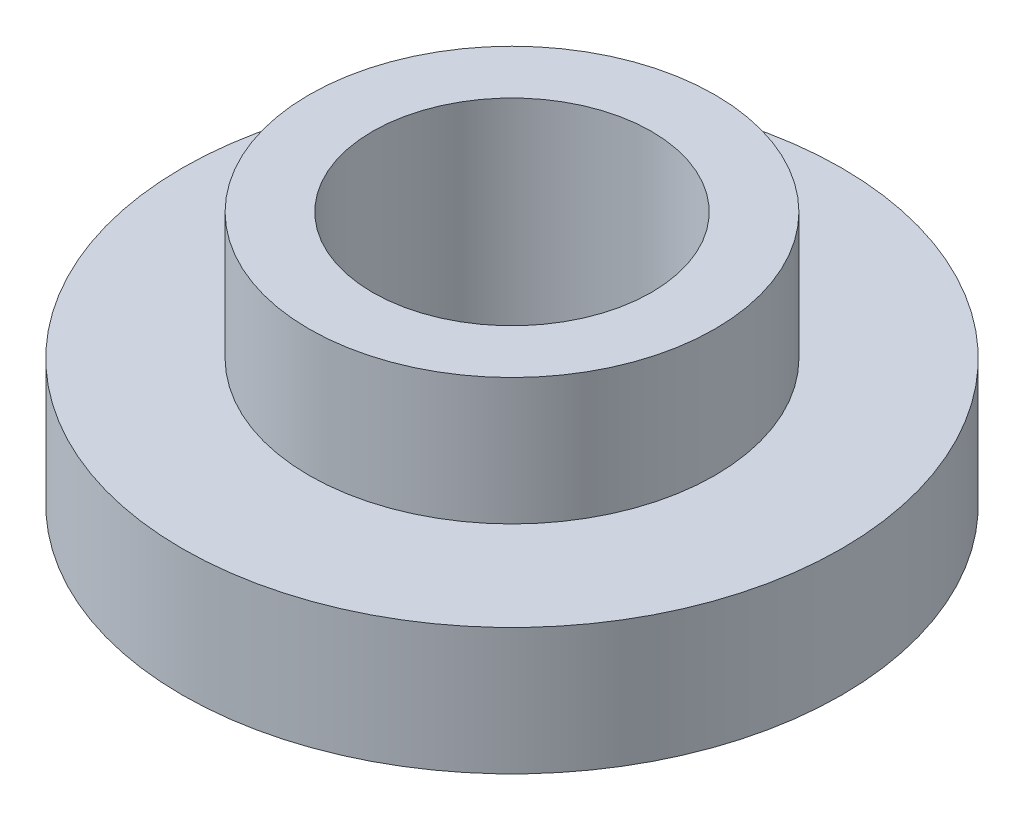
SolidWorks part; units mm, degrees
ref_plane "Front Plane" through (0, 0, 0) normal (0, 0, 1) x (1, 0, 0)
ref_plane "Top Plane" through (0, 0, 0) normal (0, 1, 0) x (1, 0, 0)
ref_plane "Right Plane" through (0, 0, 0) normal (1, 0, 0) x (0, 0, -1)
sketch "Sketch1" plane through (0, 0, 0) normal (0, 0, 1) x (1, 0, 0)
  line L0 (-29.5, 0) -> (-65, 0)
  line L1 (-65, 0) -> (-65, 25)
  line L2 (-65, 25) -> (-40, 25)
  line L3 (-40, 25) -> (-40, 50)
  line L4 (-40, 50) -> (-27.5, 50)
  line L5 (-27.5, 50) -> (-27.5, 2)
  line L6 (0, 0) -> (0, 42.4846) construction
  line L7 (0, 0) -> (-27.5, 0) construction
  line L8 (-27.5, 2) -> (-29.5, 0)
  dimension "D1" = 130
  dimension "D2" = 80
  dimension "D3" = 55
  dimension "D4" = 25
  dimension "D5" = 25
  dimension "D6" = 2
  dimension "D7" = 45
revolve "Revolve1" add sketch "Sketch1" angle 360 about L6
